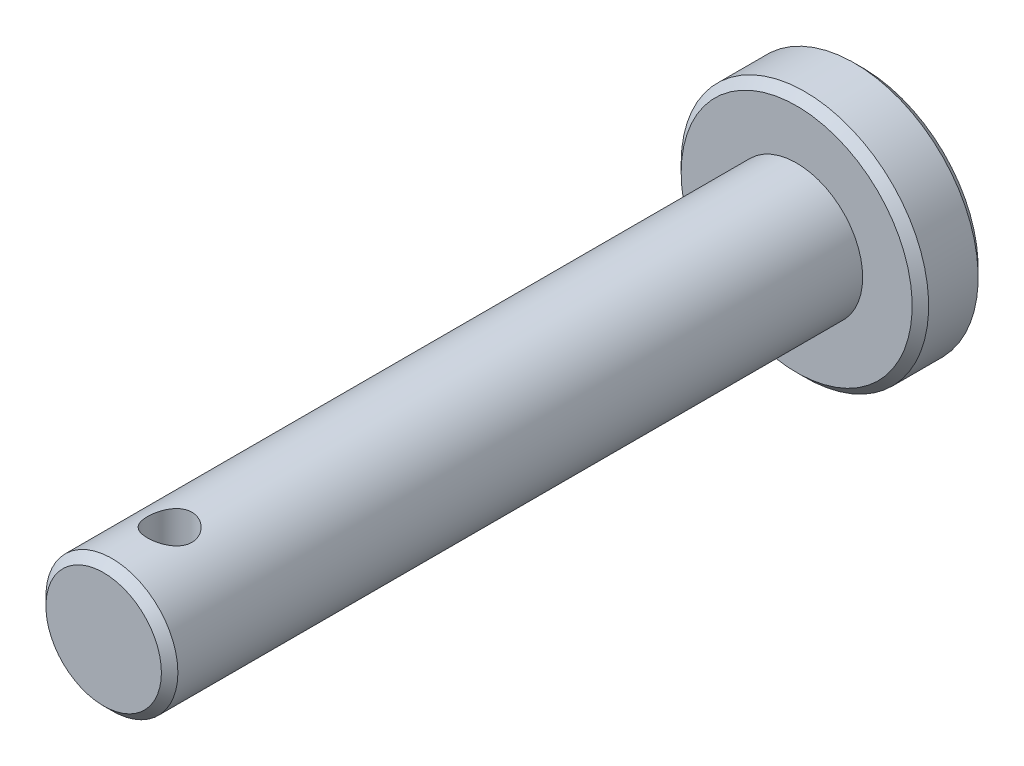
SolidWorks part; units mm, degrees
material "国产6061 "
ref_plane "Front Plane" through (0, 0, 0) normal (0, 0, 1) x (1, 0, 0)
ref_plane "Top Plane" through (0, 0, 0) normal (0, 1, 0) x (1, 0, 0)
ref_plane "Right Plane" through (0, 0, 0) normal (1, 0, 0) x (0, 0, -1)
sketch "Sketch1" plane through (0, 0, 0) normal (0, 0, 1) x (1, 0, 0)
  circle A0 centre (0, 0) radius 4
  dimension "D1" = 8
extrude "Boss-Extrude1" add sketch "Sketch1" along normal blind 42
sketch "Sketch2" plane through (0, 0, 0) normal (0, 0, -1) x (-1, 0, 0)
  circle A0 centre (0, 0) radius 7.5
  dimension "D1" = 15
extrude "Boss-Extrude2" add sketch "Sketch2" along normal blind 4
sketch "Sketch3" plane through (0, 0, 0) normal (0, 1, 0) x (1, 0, 0)
  line L0 (-4, -42) -> (4, -42) construction
  circle A0 centre (0, -38) radius 1.35
  dimension "D1" = 2.7
  dimension "D2" = 4
extrude "Cut-Extrude1" cut sketch "Sketch3" against normal through all both and the other way through all
chamfer "Chamfer1" distance 0.5 angle 45 3 edges at (4, 0, 42) (-7.5, 0, -4) (-7.5, 0, 0)
